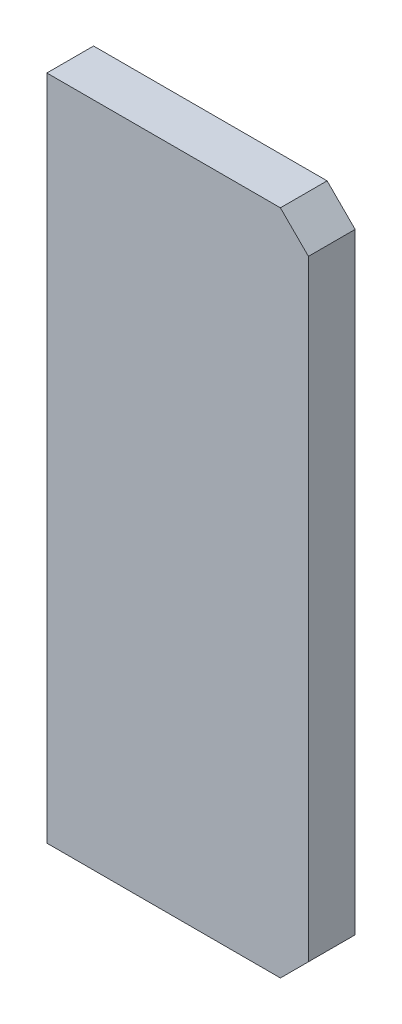
from build123d import *

# Parameters (mm, degrees)
SKETCH1_W           = 140
SKETCH1_H           = 357
BOSS_EXTRUDE1_DEPTH = 25
CHAMFER2_SIZE       = 15


with BuildPart() as part:
    # Sketch1 → Boss-Extrude1 (new body)
    with BuildSketch(Plane.XY):
        with Locations((70, 178.5)):
            Rectangle(SKETCH1_W, SKETCH1_H)
    extrude(amount=BOSS_EXTRUDE1_DEPTH)

    # Chamfer2
    chamfer2_edges = [part.edges().sort_by_distance(p)[0] for p in [
        (140, 357, 12.5),
        (140, 0, 12.5),
    ]]
    chamfer(chamfer2_edges, length=CHAMFER2_SIZE)


solid = part.part
